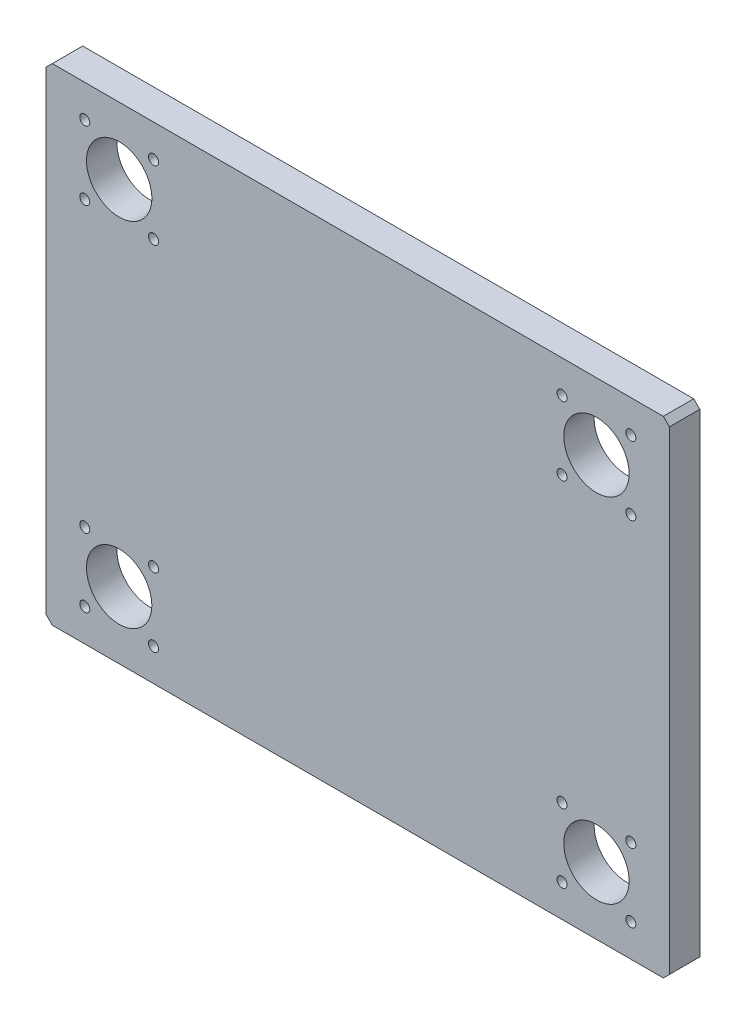
from build123d import *

# Parameters (mm, degrees)
SKETCH1_W           = 205
SKETCH1_H           = 160
BOSS_EXTRUDE1_DEPTH = 10
SKETCH2_R           = 10.75
CUT_EXTRUDE1_DEPTH  = 131.408013557
M4_TAPPED_HOLE1_D   = 3.3
CHAMFER1_SIZE       = 2


with BuildPart() as part:
    # Sketch1 → Boss-Extrude1 (new body)
    with BuildSketch(Plane.XY):
        Rectangle(SKETCH1_W, SKETCH1_H)
    extrude(amount=BOSS_EXTRUDE1_DEPTH)

    # Sketch2 → Cut-Extrude1 (cut, through all)
    with BuildSketch(Plane.XY.offset(10)):
        with Locations((-78.5, -58)):
            Circle(SKETCH2_R)
        with Locations(Location((-78.5, 58, 0), (0, 0, 180))):
            Circle(SKETCH2_R)
        with Locations(Location((78.5, -58, 0), (0, 0, 180))):
            Circle(SKETCH2_R)
        with Locations((78.5, 58)):
            Circle(SKETCH2_R)
    extrude(amount=-CUT_EXTRUDE1_DEPTH, mode=Mode.SUBTRACT)

    # M4 Tapped Hole1 (through all)
    with Locations(Plane.XY.offset(10)):
        with Locations((-89.813708499, 69.313708499), (-67.186291501, 69.313708499), (-67.186291501, 46.686291501), (-89.813708499, 46.686291501), (67.186291501, 69.313708499), (89.813708499, 69.313708499), (67.186291501, 46.686291501), (89.813708499, 46.686291501), (-89.813708499, -46.686291501), (-67.186291501, -46.686291501), (-89.813708499, -69.313708499), (-67.186291501, -69.313708499), (67.186291501, -46.686291501), (89.813708499, -46.686291501), (67.186291501, -69.313708499), (89.813708499, -69.313708499)):
            Hole(M4_TAPPED_HOLE1_D / 2)

    # Chamfer1
    chamfer1_edges = [part.edges().sort_by_distance(p)[0] for p in [
        (102.5, -80, 5),
        (-102.5, -80, 5),
        (-102.5, 80, 5),
        (102.5, 80, 5),
    ]]
    chamfer(chamfer1_edges, length=CHAMFER1_SIZE)


solid = part.part
